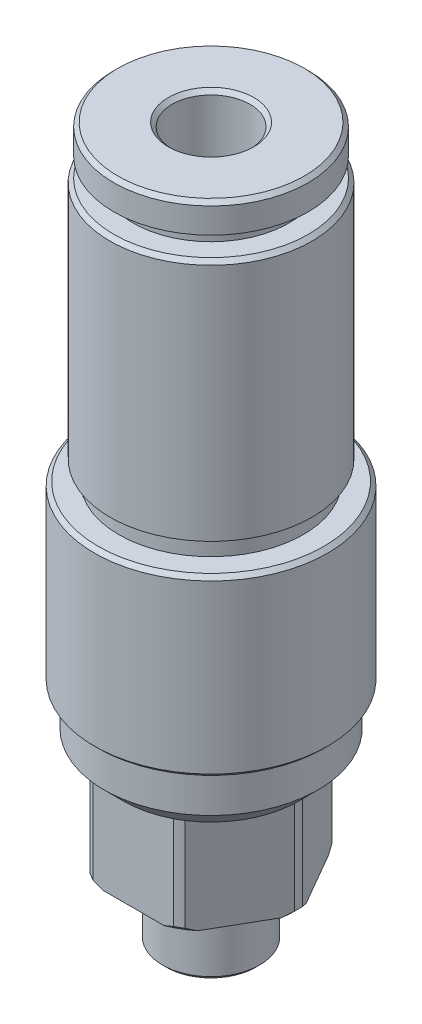
from build123d import *

# Parameters (mm, degrees)
SKETCH3_OUTSIDE_W  = 22.05
SKETCH3_OUTSIDE_H  = 22.05
CUT_EXTRUDE1_DEPTH = 5


with BuildPart() as part:
    # Sketch1 → Revolve1 (revolve)
    with BuildSketch(Plane.XY, mode=Mode.PRIVATE) as revolve1_sk:
        Polygon((1.45, 0), (2.3, 0), (2.5, 0.2), (2.5, 3), (2, 3), (2, 3.5), (4.3, 3.5), (4.5, 3.7), (4.5, 8.5), (5.5, 9.5), (5.5, 11.5), (5.8, 11.5), (6, 11.7), (6, 20.3), (5.8, 20.5), (4.75, 20.5), (4.75, 21.5), (5.2, 21.5), (5.2, 33.8), (5, 34), (4, 34), (4, 35), (5, 35), (5, 36.3), (4.8, 36.5), (2.2, 36.5), (2, 36.3), (2, 5.75), (1.25, 5), (1.25, 0.2), align=None)
    revolve(revolve1_sk.sketch.rotate(Axis((0, 0, 0), (0, 1, 0)), 90), axis=Axis((0, 0, 0), (0, 1, 0)))

    # Sketch3 outside → Cut-Extrude1 (cut)
    with BuildSketch(Plane.XZ.offset(-3.5)):
        Rectangle(SKETCH3_OUTSIDE_W, SKETCH3_OUTSIDE_H)
        Polygon((2.309401077, -4), (4.618802154, 0), (2.309401077, 4), (-2.309401077, 4), (-4.618802154, 0), (-2.309401077, -4), align=None, mode=Mode.SUBTRACT)
    extrude(amount=-CUT_EXTRUDE1_DEPTH, mode=Mode.SUBTRACT)


solid = part.part
